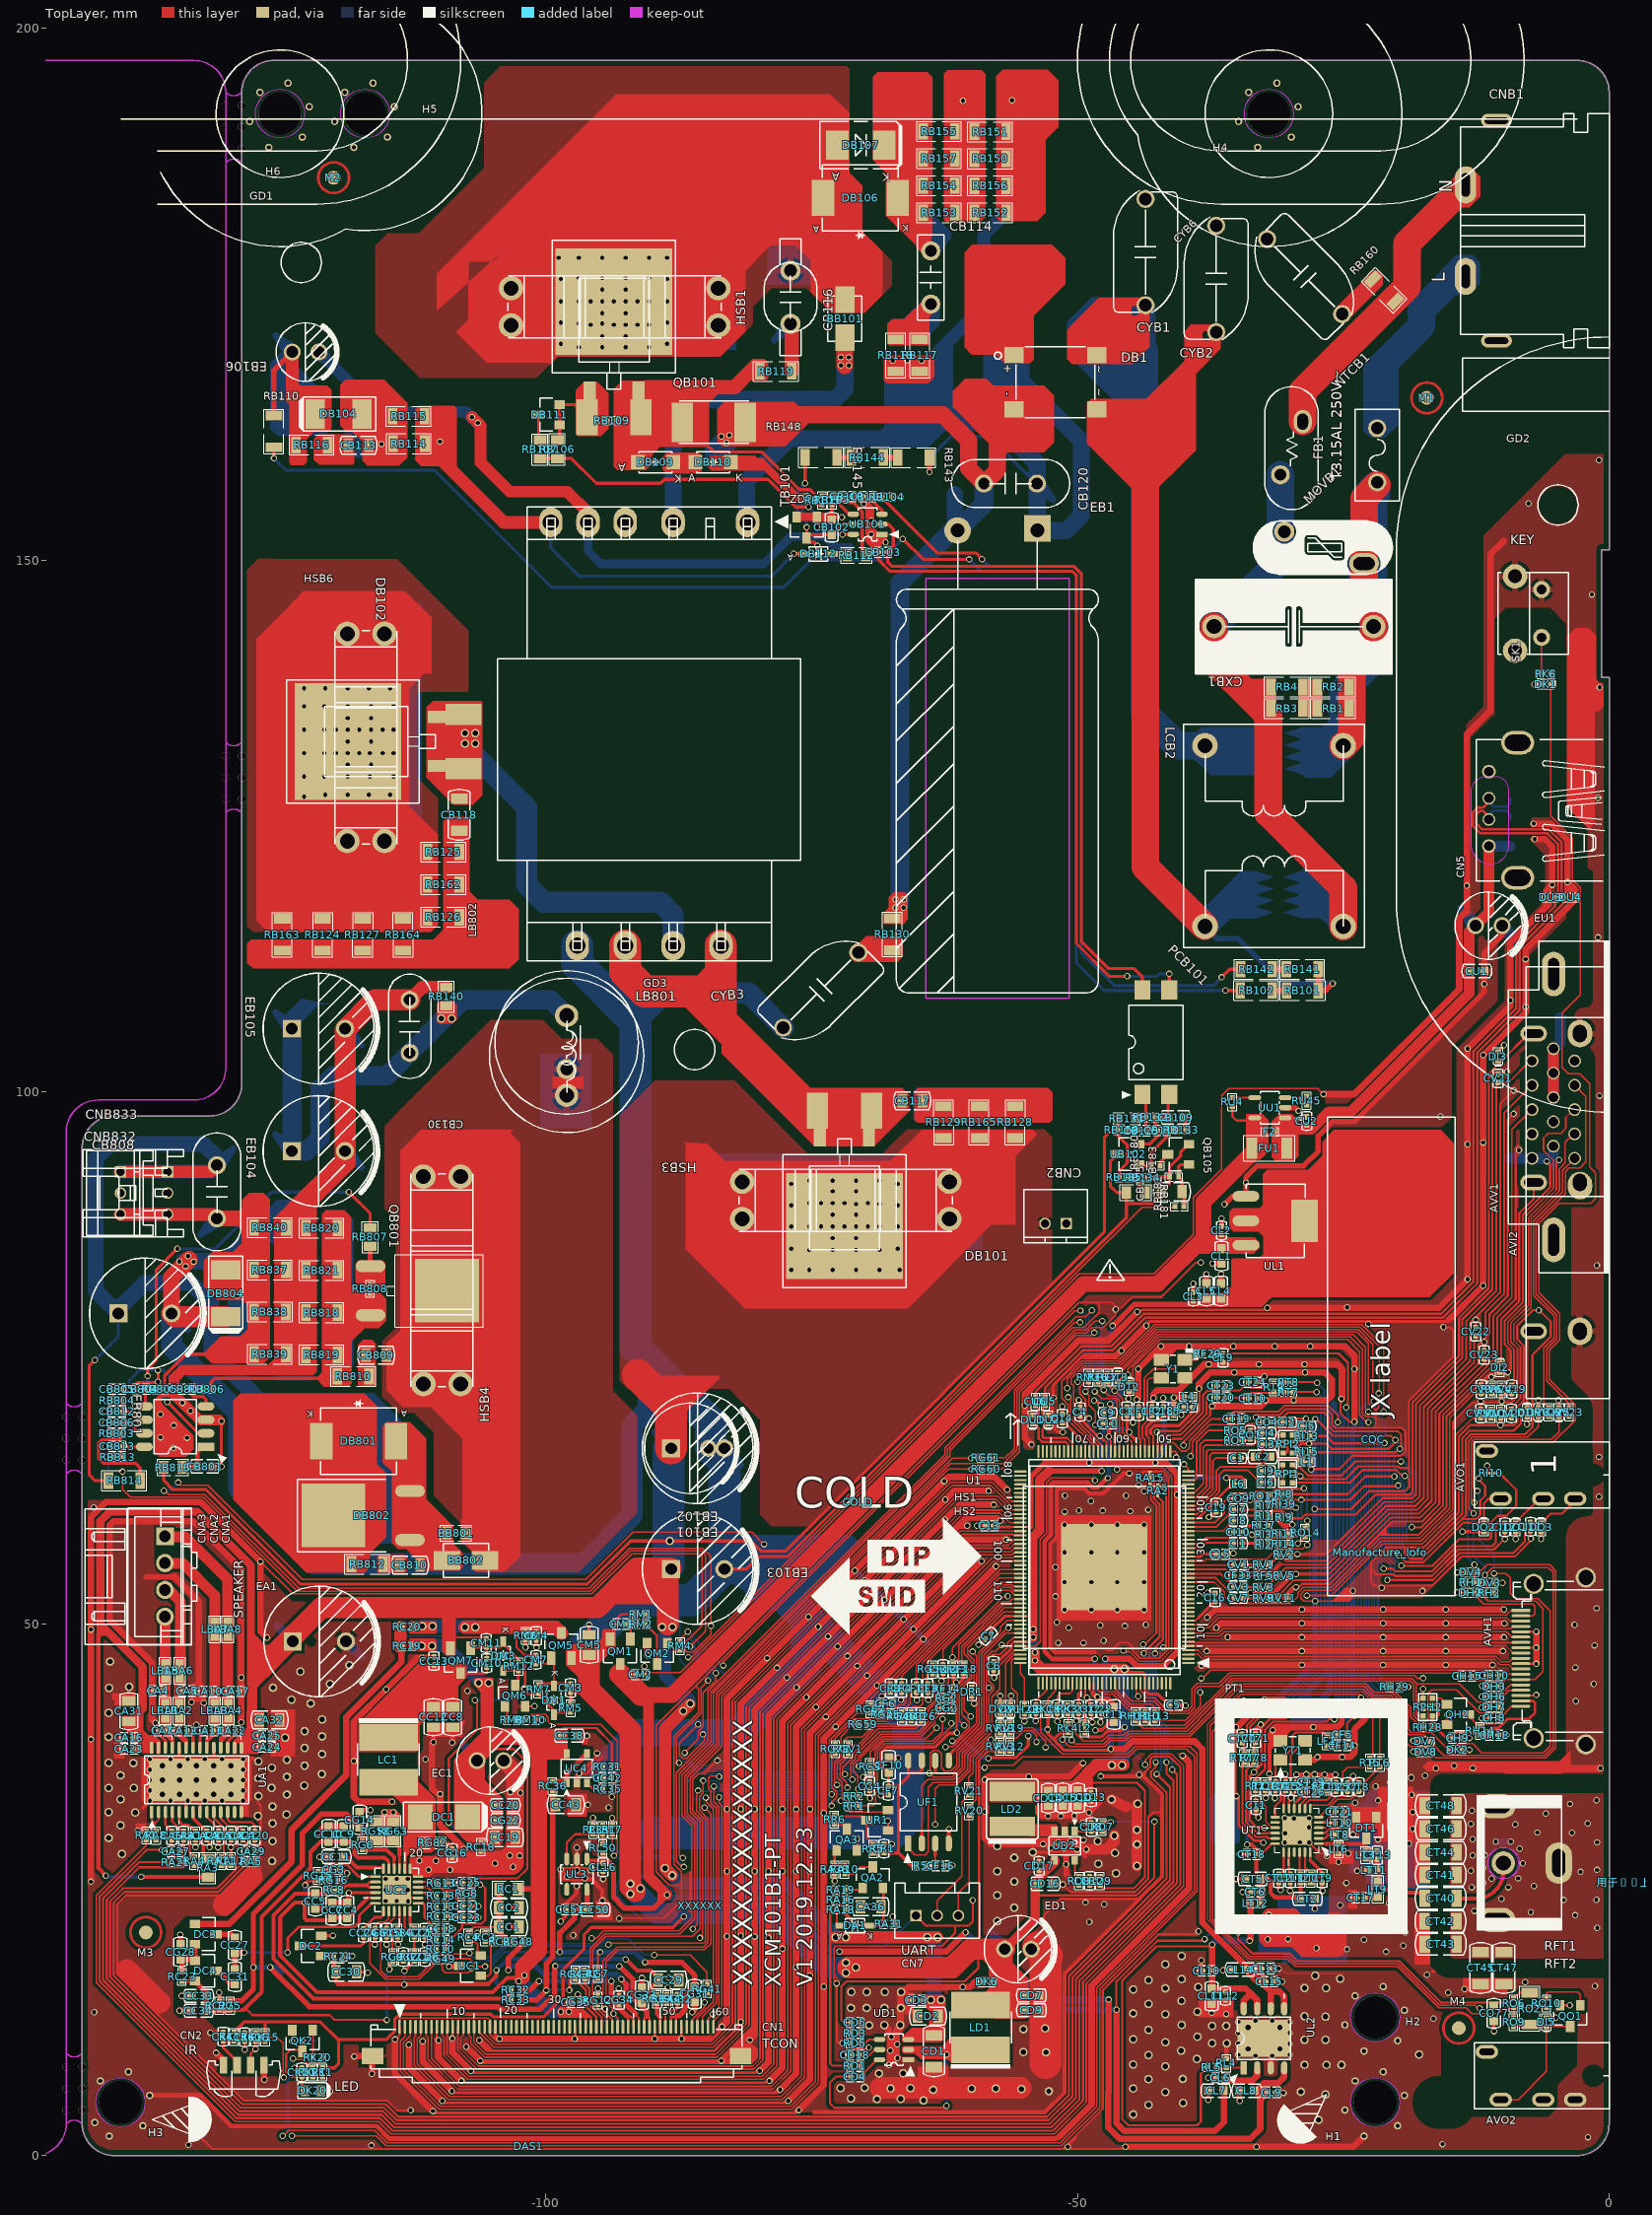
[diagram p0: TopLayer view]
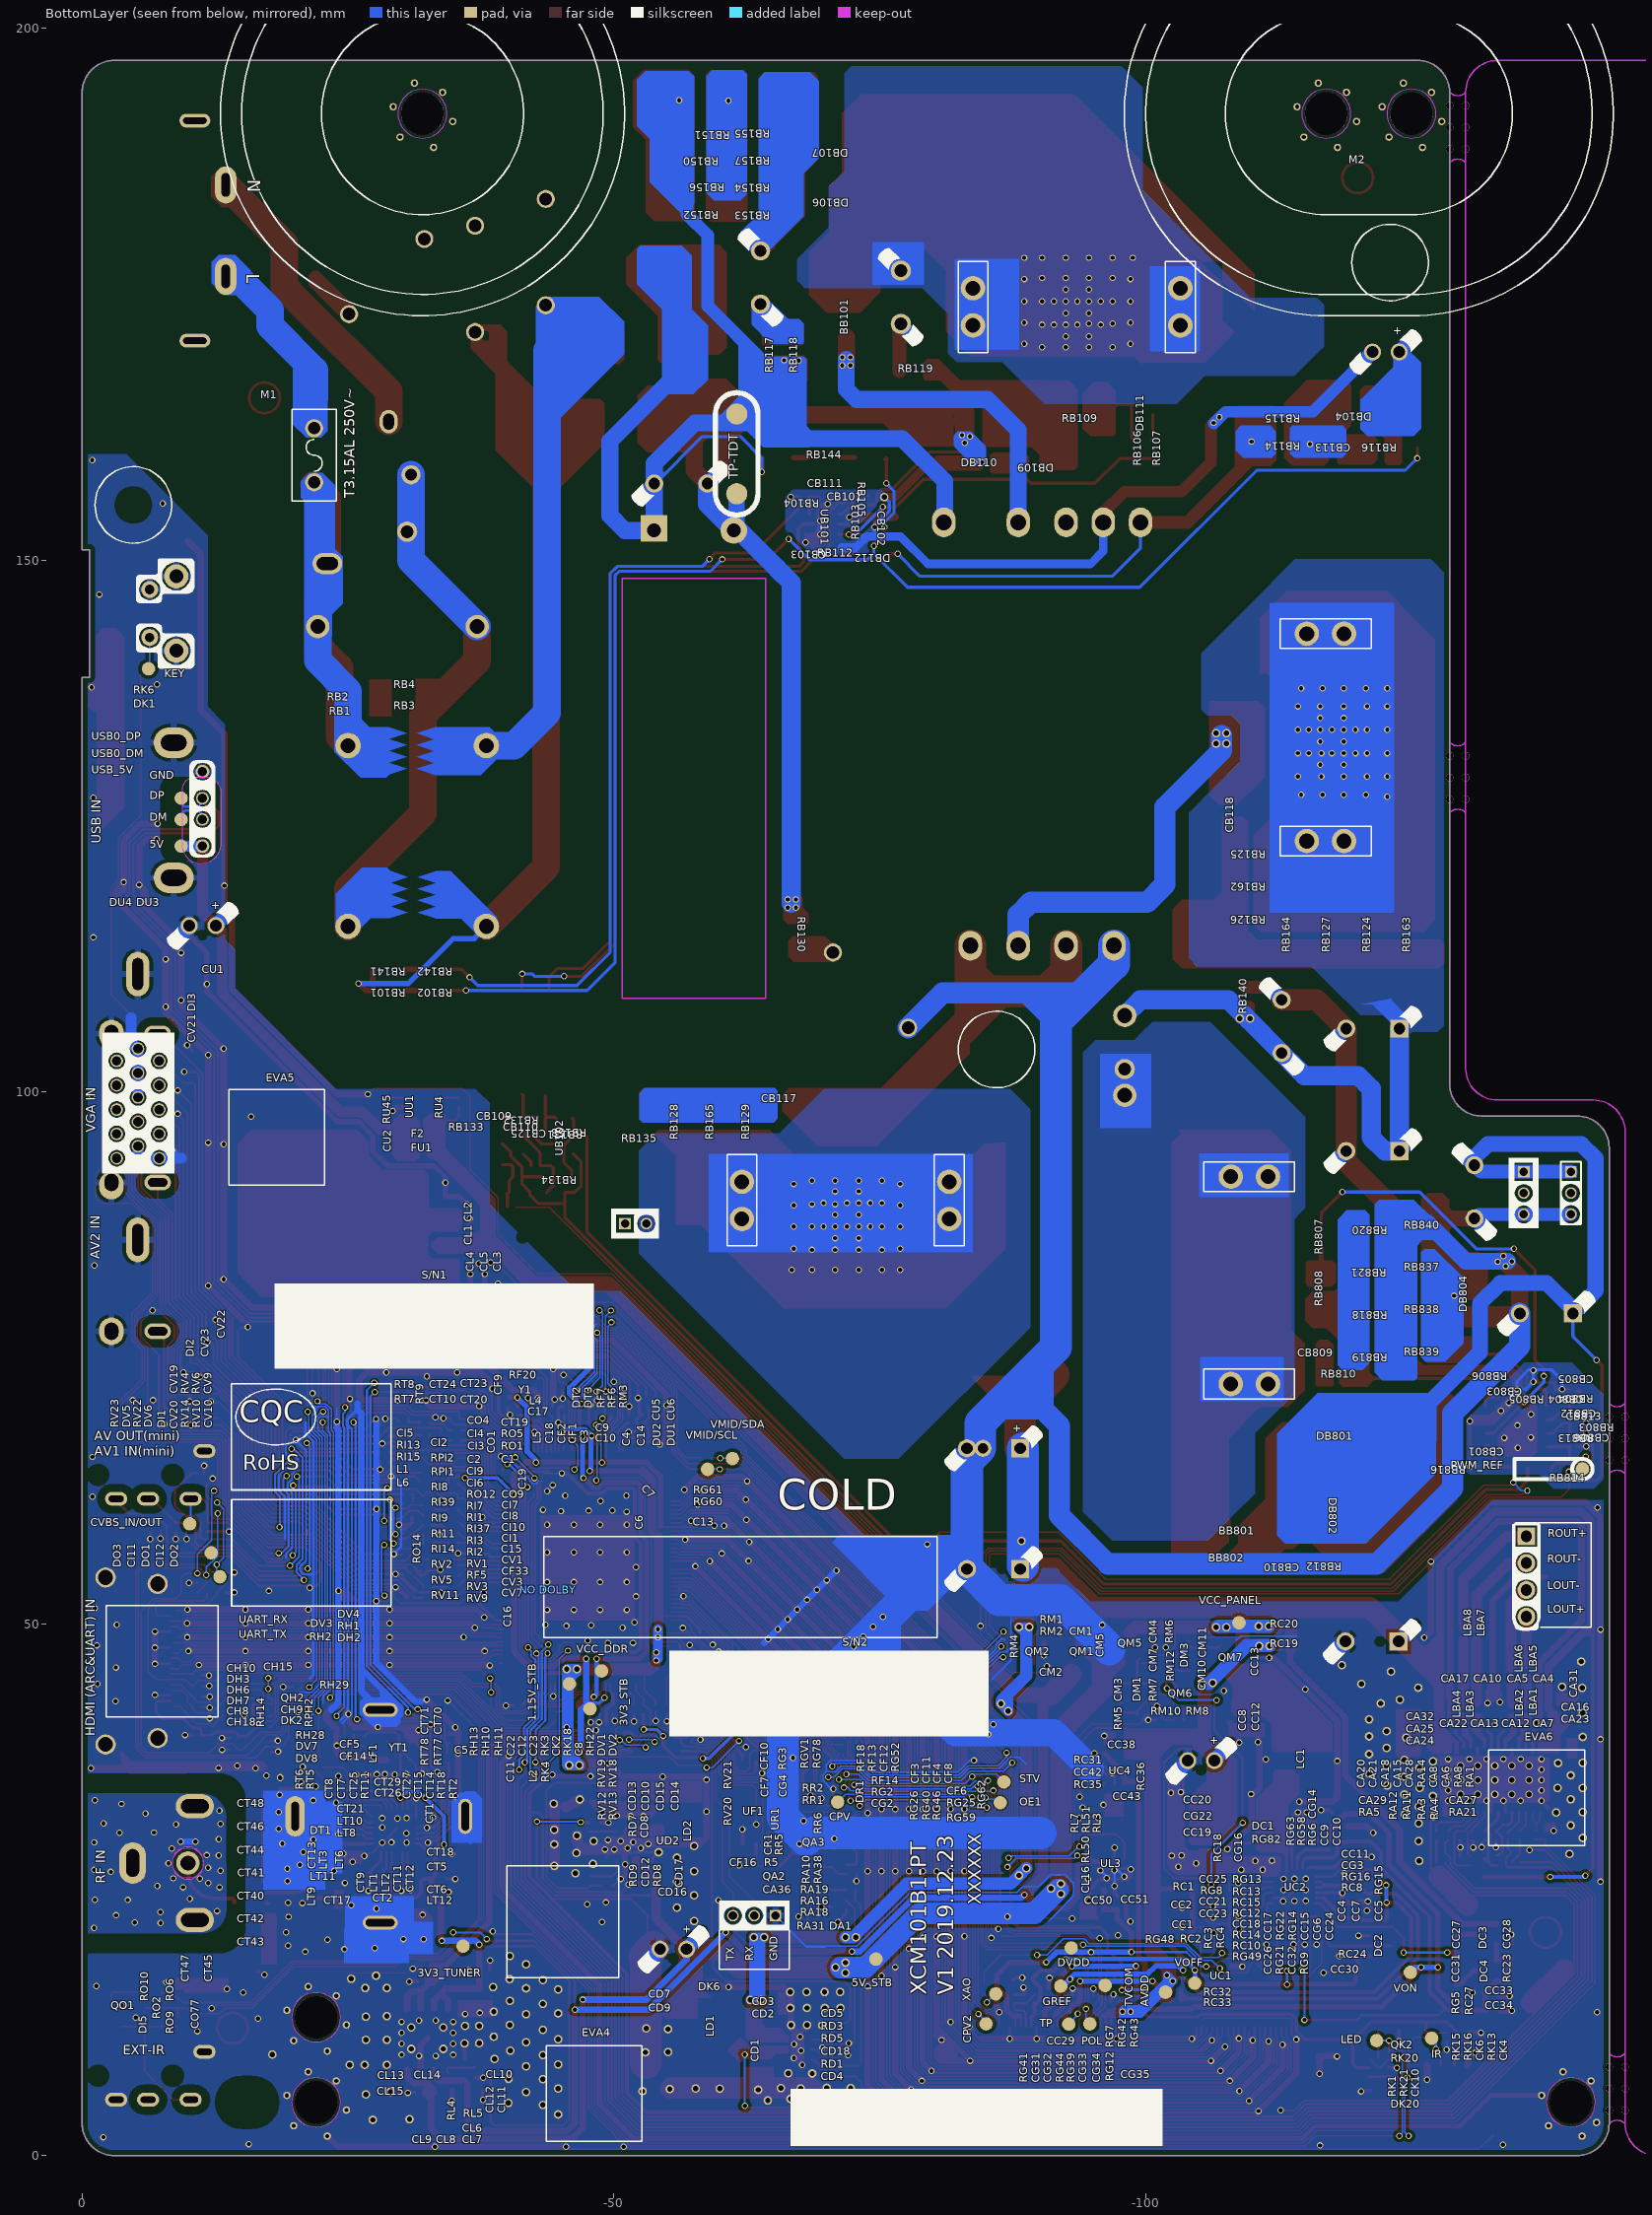
[diagram p1: BottomLayer view, seen from below]
# Altium PCB MISC86383-9.PcbDoc (part 1 of 18)
Units mm, origin at the board's own origin, x right, y up, seen from the top; angles counter-clockwise.
Board outline 143.6 x 197 mm, 2 copper layers (TopLayer, BottomLayer), stack 1.571 mm thick; 743 components, 401 nets, 2996 pads, 1077 vias.
Unrouted connection lines stored in the file: 4.

## Layer stack, top to bottom
TopSolder: solder mask 0.0102, Solder Resist, Dk 3.5
TopLayer: signal copper 0.0356
Dielectric1: core 1.5, FR-4, Dk 4.8
BottomLayer: signal copper 0.0356
BottomSolder: solder mask 0.0102, Solder Resist, Dk 3.5

## Board outline
-140.6,0 cw(c-140.6,3) -143.6,3 -143.6,94.75 cw(c-140.6,94.75) -140.6,97.75 -131.6,97.75 ccw(c-131.6,100.75) -128.6,100.75 -128.6,194 cw(c-125.6,194) -125.6,197 -3,197 cw(c-3,194) 0,194 0,151 -0.7,151 -0.7,139 0,139 0,3 cw(c-3,3) -3,0

## Design rules (kind name [scope] priority, off if disabled: settings)
Clearance ■KEEPOUT_18mil [(IsTrack Or IsArc) And (AsMM(Width) < 1) And IsKeepOut vs Not IsPad] p1: gap=0.457
Clearance ■HOT_8mm [InNetClass('HOT') vs InNetClass('All Nets') And (Not InNetClass('HOT'))] p2: gap=8
Clearance ■DFM_NPTH_10mil [(IsPadHoleValid And (PadIsPlated=false) Or IsPad And ((AsMM(PadXSize_AllLayers) < 1) or (AsMM(PadYSize_AllLayers) < 1 )) And IsKeepout) OR HasFootprintPad('ASSE*','0') vs Not IsPad] p3: gap=0.254
Clearance ■DFM_20mil [(IsTrack or IsArc or IsPad) And IsKeepOut vs IsTrack or IsArc or InPoly] p4: gap=0.508
Clearance ■C_RJ45_2mm [InNetClass('RJ45') vs Not InNetClass('RJ45') AND InNet('*')] p5: gap=2
Clearance ■VIA2VIA_6.2mil [(IsVia OR InPadClass('VIA5')) And Not ((IsVia OR InPadClass('VIA5')) And (AsMM(HoleDiameter) = 0.1)) vs (IsVia OR InPadClass('VIA5')) And Not ((IsVia OR InPadClass('VIA5')) And (AsMM(HoleDiameter) = 0.1))] p6: gap=0.157
Clearance ■V2V_BGA0p65_9p8mil [((IsVia OR InPadClass('VIA5')) And Not ((IsVia OR InPadClass('VIA5')) And (AsMM(HoleDiameter) = 0.1))) And (WithInRoom('BGA0p65-1') OR WithInRoom('BGA0p65-2')) vs ((IsVia OR InPadClass('VIA5')) And Not ((IsVia OR InPadClass('VIA5')) And (AsMM(HoleDiameter) = 0.1))) And (WithInRoom('BGA0p65-1') OR WithInRoom('BGA0p65-2'))] p7: gap=0.249
Clearance ■VIA2VIA_10.2mil [((IsVia OR InPadClass('VIA5')) And Not ((IsVia OR InPadClass('VIA5')) And (AsMM(HoleDiameter) = 0.1))) And Not (WithInRoom('BGA0p65-1') OR WithInRoom('BGA0p65-2')) vs ((IsVia OR InPadClass('VIA5')) And Not ((IsVia OR InPadClass('VIA5')) And (AsMM(HoleDiameter) = 0.1))) And Not (WithInRoom('BGA0p65-1') OR WithInRoom('BGA0p65-2'))] p8: gap=0.259
Clearance 0.3mm [(InNet('VGH') or InNet('*VGHM*')) and Not IsPad vs Not InPoly] p9: gap=0.3
Clearance ■PWR_A12_8mil [((InNetClass('PWR_A12_8mil') or InNet('*12V*') or InNet('*24V*') or InNet('AVDD') or InNet('*PVCC*') or InNet('*19V*') or InNet('*AMP*POWER*') or InNet('*AMP*VCC*') or InNet('*LNB*')) And Not InNetClass('A12_8mil_EXC')or InNet('VDD1')or InNet('VDD2')or InNet('CLK6')or InNet('CLK5')or InNet('CLK4')or InNet('CLK3')or InNet('CLK2')or InNet('CLK1')or InNet('DRVN')or InNet('DRVP')) and Not IsPad vs Not InPoly] p10: gap=0.203
Clearance ■PS_L2All_3.2mm [InNet('L-1') vs InNet('*')] p11: gap=3.2
Clearance ■PS_L2LN_1.5mm [InNet('L') Or InNet('L-2') Or InNet('L-3') Or InNet('L-4') Or InNet('L-5') Or InNet('L-6') vs InNet('L-N') And Not(InNet('L') Or InNet('L-2') Or InNet('L-3') Or InNet('L-4') Or InNet('L-5') Or InNet('L-6'))] p12: gap=1.5
Clearance ■PS_N2LN_1.5mm [InNet('N') OR InNet('N-1') OR InNet('N-2') OR InNet('N-3') OR InNet('N-4') OR InNet('N-5') OR InNet('N-6') vs InNet('L-N') And Not (InNet('N') OR InNet('N-1') OR InNet('N-2') OR InNet('N-3') OR InNet('N-4') OR InNet('N-5') OR InNet('N-6'))] p13: gap=1.5
Clearance ■PS_L2LN_3.1mm [InNet('L') Or InNet('L-2') Or InNet('L-3') Or InNet('L-4') Or InNet('L-5') Or InNet('L-6') vs InNet('*') And Not (InNet('L-N') Or InNet('L') Or InNet('L-2') Or InNet('L-3') Or InNet('L-4') Or InNet('L-5') Or InNet('L-6') Or OnLayer('KeepOutLayer'))] p14: gap=3.1
Clearance ■PS_N2LN_3.1mm [InNet('N') OR InNet('N-1') OR InNet('N-2') OR InNet('N-3') OR InNet('N-4') OR InNet('N-5') OR InNet('N-6') vs InNet('*') And Not (InNet('L-N') Or InNet('N') OR InNet('N-1') OR InNet('N-2') OR InNet('N-3') OR InNet('N-4') OR InNet('N-5') OR InNet('N-6') Or OnLayer('KeepOutLayer'))] p15: gap=3.1
Clearance 2.1mm [InNet('VBRIDGE')  Or InNet('D_QB101') vs InNet('*')And Not InNet('VBRIDGE')  And Not InNet('D_QB101')] p16: gap=2.1
Clearance 0.5mm [InNet('VBL')  Or InNet('LED+') Or InNet('D_QB801') vs InNet('*')And Not InNet('VBL')  And Not InNet('LED+')And Not InNet('D_QB801')] p17: gap=0.5
Clearance ■SIP2GND_8mil [HasFootprint('SIP*') vs InPoly] p18: gap=0.203
Clearance ■C_BGA_0P65 [HasFootprint('BGA*0.65*') vs InPoly] p19: gap=0.127
Clearance ■C_BGA_0P8 [HasFootprint('BGA*0.8*') vs InPoly] p20: gap=0.14
Clearance ■Poly_4mil [InPolygonClass('Poly_4mil') vs Not InPoly] p21: gap=0.102
Clearance ■Poly_5mil [InPolygonClass('Poly_5mil') vs Not InPoly] p22: gap=0.127
Clearance ■Poly_6.2mil [InPolygonClass('Poly_6.2mil') vs Not InPoly] p23: gap=0.157
Clearance Poly_7mil [InPolygonClass('Poly_7mil') vs Not InPoly] p24: gap=0.178
Clearance ■Poly_8mil [InPolygonClass('Poly_8mil') vs Not InPoly] p25: gap=0.203
Clearance ■C_RFGND_1.8mm [InNet('RFGND') vs Not (InNet('RF*IN*') OR((IsTrack Or IsArc) And (AsMils(Width) < 6) And IsKeepOut) OR InNet('NetCT28*'))] p26: gap=1.8
Clearance ■ESD_10mil [HasFootprint('*IEC*') Or HasFootprint('*-F1*') Or HasFootprint('ANT-RF*')] p27: gap=0.254
Clearance ■ESD_20mil [HasFootprint('*SHIELD*')] p28: gap=0.508
Clearance ■GND_12mil [InNet('GND') vs InPoly] p29: gap=0.305
Clearance ■ESD_30mil [(HasFootprint('SCART*') OR HasFootprint('AV*') OR HasFootprint('DB15*') OR HasFootprint('PHONE*')) vs OnBottomLayer] p30: gap=0.762
Clearance ■ESD_NT_30mil [HasFootprint('SCART*') Or HasFootprint('PHONE-HD-12') Or HasFootprint('PHONE-HD-17') Or HasFootprint('PHONE-HD-10') Or HasFootprint('PHONE-HD-26') vs InNet('GND') And OnTopLayer] p31: gap=0.762
Clearance ■DFM_TH_5mil [HasFootprint('GND') or HasFootprint('TP*') or HasFootprint('MARK*') or HasFootprint('SPARK_GAP') or HasFootprint('USB-HD-3-2') or HasFootprint('PHONE-HS-20') and Not IsRegion vs OnBottomlayer And IsPad OR IsPadHoleValid] p32: gap=0.127
Clearance ■DFM_HS60_5mil [InPadClass('HS60') vs InPadClass('HS60') OR IsPadHoleValid and not InPadClass('VIA5')] p33: gap=0.127
Clearance ■DFM_BCR_4mm [IsPadHoleValid vs IsBoardCutoutRegion] p34: gap=4
Clearance ■DFM_TH_4mm [OnBottomlayer And IsSMTPin vs IsPadHoleValid and not InPadClass('VIA5')] p35: gap=4
Clearance ■DFM_HS60_4mm [InPadClass('HS60') vs IsPad and OnBottomlayer] p36: gap=4
Clearance ■V2P_BGA0p65_4p7mil [HasFootprint('BGA*') and IsPad And (WithInRoom('BGA0p65-1') OR WithInRoom('BGA0p65-2')) vs (IsVia OR InPadClass('VIA5')) And Not (IsVia And (AsMM(HoleDiameter) = 0.1))] p37: gap=0.119
Clearance ■VIA2PAD_BGA_5mil [(HasFootprint('BGA*') and IsPad) And Not (WithInRoom('BGA0p65-1') OR WithInRoom('BGA0p65-2')) vs (IsVia OR InPadClass('VIA5')) And Not (IsVia And (AsMM(HoleDiameter) = 0.1))] p38: gap=0.127
Clearance ■VIA2PAD_6mil [(IsVia OR InPadClass('VIA5')) And Not ((IsVia OR InPadClass('VIA5')) And (AsMM(HoleDiameter) = 0.1)) vs IsPad And Not HasFootprintPad('*','EPAD') and Not HasFootprintPad('*','257') and Not HasFootprintPad('TP','*') and Not HasFootprintPad('GND','JP*') and Not HasFootprintPad('LQFP216/0.4-2','217') and Not HasFootprintPad('QFP16*','17') and Not HasFootprintPad('QFN16*','17') and Not HasFootprintPad('QFN20*','21') and Not HasFootprintPad('QFN24*','25') and Not HasFootprintPad( 'QFN24*','29') and Not HasFootprintPad('QFN28*','29') and Not HasFootprintPad('QFN32*','33') and Not HasFootprintPad('QFN36*','37') and Not HasFootprintPad('QFN36*','0') and Not HasFootprintPad('QFN32*','0') and Not HasFootprintPad('QFN40*','41') and Not HasFootprintPad('QFN48*','49') and Not HasFootprintPad('LQFP48/0.5-2','49') and Not HasFootprintPad('*SSOP32*','33') and Not HasFootprintPad('SOP8*','9') and Not HasFootprintPad('WSON8/1.27*','9') and Not HasFootprintPad('DFN10/0.5-1*','11') and Not HasFootprintPad('SON16/0.4','9') and Not HasFootprintPad('MSOP10/0.5-1','11') and Not HasFootprintPad('QFN56/0.5','57') and Not HasFootprintPad('LGA31/0.5','3*') and Not InPadClass('VIA_HS60') and Not HasFootprintPad('TSSOP16/0.65-3','17') and Not HasFootprintPad('QFP128/0.5-2','129') and Not HasFootprintPad('QFP128/0.4-5','129') and Not HasFootprintPad('PQFP48*','49') and Not HasFootprintPad('QFP156/0.4-1','157') and Not HasFootprintPad('D2PAK3-TO-252','2') and Not HasFootprintPad('D2PAK3','2') and Not HasFootprintPad('TO-252-GDS','D')  and Not HasFootprintPad('TO-252','2')  and Not HasFootprintPad('QFP156/0.4-2','157')] p39: gap=0.152
Clearance ■PAD2VIA5_6mil [(IsPad And Not (WithInRoom('BGA0p65-1') OR WithInRoom('BGA0p65-2'))) And ((AsMM(PadXSize_AllLayers) < 2.5) or ((AsMM(PadYSize_AllLayers) < 2.5))) And Not InPadclass('HS60') vs InPadClass('VIA5')] p40: gap=0.152
Clearance "■12mil for Polygon" [InPoly] p41: gap=0.305
Clearance 8mil [All] p42 off: gap=0.203
Clearance 7mil [All] p43 off: gap=0.178
Clearance 6.2mil [All] p44 off: gap=0.157
Clearance 6mil [All] p45 off: gap=0.152
Clearance 5.8mil [All] p46 off: gap=0.147
Clearance 5mil [Not ((IsTrack Or IsArc) And (Layer = 'KeepOutLayer')) vs Not (IsPad or ((IsTrack Or IsArc) And (Layer = 'KeepOutLayer')))] p47: gap=0.127
Clearance 4.5mil [Not ((IsTrack Or IsArc) And (Layer = 'KeepOutLayer')) vs Not (IsPad or ((IsTrack Or IsArc) And (Layer = 'KeepOutLayer')))] p48 off: gap=0.114
Clearance "4mil for Minimum" [Not ((IsTrack Or IsArc) And (Layer = 'KeepOutLayer')) vs Not (IsPad or ((IsTrack Or IsArc) And (Layer = 'KeepOutLayer')))] p49 off: gap=0.102
ComponentClearance ■DFMC_1mm [Not (InComponentClass('Co-Layout') Or HasFootprint('GND')) And (HasFootprint('T/E*') Or HasFootprint('T/PQ*') Or HasFootprint('USB*') Or HasFootprint('HDMI*') Or HasFootprint('USB*') Or HasFootprint('DC-*') Or HasFootprint('AV*') Or HasFootprint('ANT*') Or HasFootprint('PHONE*') Or HasFootprint('CICARD*') Or HasFootprint('CARD*') Or HasFootprint('DVI*') Or HasFootprint('DB*') Or HasFootprint('DP*') Or HasFootprint('DISPLAYPORT*') Or HasFootprint('OPTICAL*') Or HasFootprint('SCART*') Or HasFootprint('RJ45*') Or HasFootprint('USB*') Or HasFootprint('T-*') Or HasFootprint('T/*') Or HasFootprint('200-*') Or HasFootprint('ZhiJia*') Or HasFootprint('Dianpian*') Or HasFootprint('TanPian*') Or HasFootprint('P(*')) vs Not (InComponentClass('Co-Layout') Or HasFootprint('GND'))] p1 off: gap=1 collisioncheckmode=3 verticalgap=1 showdistances=FALSE
ComponentClearance ■DFMC_0.5mm [Not (InComponentClass('Co-Layout') Or HasFootprint('SO-23') Or HasFootprint('DIODE-s0402') Or HasFootprint('GND')) And (HasFootprint('M-*') Or HasFootprint('BGA*') Or HasFootprint('QFP*') Or HasFootprint('QFN*') Or HasFootprint('*DFN*') Or HasFootprint('*SOP*') Or HasFootprint('LGA*') Or HasFootprint('SOIC*') Or HasFootprint('EC*') Or HasFootprint('AC-*') Or HasFootprint('DIODE*') Or HasFootprint('XTAL*') Or HasFootprint('SO-*') Or HasFootprint('L/LC*') Or HasFootprint('L(*') Or HasFootprint('WIFI*') Or HasFootprint('SATA*') Or HasFootprint('POGO*') Or HasFootprint('SOT-223') Or HasFootprint('TO-252') Or HasFootprint('TO-263') Or HasFootprint('KEY*') Or HasFootprint('SW*') Or HasFootprint('DIP*') Or HasFootprint('SIP*') Or HasFootprint('DIP*') Or HasFootprint('CON*') Or HasFootprint('FFC*') Or HasFootprint('FPC*') Or HasFootprint('GDT*') Or HasFootprint('R2512*') Or HasFootprint('R2725*') Or HasFootprint('L2012*') Or HasFootprint('L2520*')) vs Not (InComponentClass('Co-Layout') Or HasFootprint('SO-23') Or HasFootprint('DIODE-s0402') Or HasFootprint('GND'))] p2 off: gap=0.5 collisioncheckmode=3 verticalgap=0.5 showdistances=FALSE
ComponentClearance ■DFMC_0.4mm [Not (InComponentClass('Co-Layout') Or HasFootprint('GND')) And (HasFootprint('C0201*') Or HasFootprint('C0402*') Or HasFootprint('C0603*') Or HasFootprint('C0805*') Or HasFootprint('C1206*') Or HasFootprint('C1210*') Or HasFootprint('R0201*') Or HasFootprint('R0402*') Or HasFootprint('R0603*') Or HasFootprint('R0805*') Or HasFootprint('R*0402*') Or HasFootprint('L0201*') Or HasFootprint('L0402*') Or HasFootprint('L0603*') Or HasFootprint('L0805*') Or HasFootprint('L1206*') Or HasFootprint('DIODE-s0402')) vs Not (InComponentClass('Co-Layout') Or HasFootprint('GND')) And (HasFootprint('C0201*') Or HasFootprint('C0402*') Or HasFootprint('C0603*') Or HasFootprint('C0805*') Or HasFootprint('C1206*') Or HasFootprint('C1210*') Or HasFootprint('R0201*') Or HasFootprint('R0402*') Or HasFootprint('R0603*') Or HasFootprint('R0805*') Or HasFootprint('R*0402*') Or HasFootprint('L0201*') Or HasFootprint('L0402*') Or HasFootprint('L0603*') Or HasFootprint('L0805*') Or HasFootprint('L1206*') Or HasFootprint('DIODE-s0402'))] p3 off: gap=0.4 collisioncheckmode=3 verticalgap=0.4 showdistances=FALSE
ComponentClearance ■DFMC_0.36mm [Not (InComponentClass('Co-Layout') Or HasFootprint('GND')) And HasFootprint('R1206*') vs Not (InComponentClass('Co-Layout') Or HasFootprint('GND')) And HasFootprint('R1206*')] p4 off: gap=0.36 collisioncheckmode=3 verticalgap=0.36 showdistances=FALSE
ComponentClearance ■DFMC_0.25mm [Not (InComponentClass('Co-Layout') Or HasFootprint('GND')) vs Not (InComponentClass('Co-Layout') Or HasFootprint('GND'))] p5 off: gap=0.25 collisioncheckmode=3 verticalgap=0.25 showdistances=FALSE
DiffPairsRouting ■DiffPair_USB_DiffPairsRouting [InDifferentialPairClass('USB')] p1: maxlimit=0.127 minlimit=0.102 mostfreqgap=0.127 toplayer_minwidth=0.381 toplayer_maxwidth=0.381 toplayer_prefwidth=0.381 bottomlayer_minwidth=0.381 bottomlayer_maxwidth=0.381 bottomlayer_prefwidth=0.381 maxuncoupledlength=5.08
DiffPairsRouting ■DiffPair_LVDS_DiffPairsRouting [InDifferentialPairClass('LVDS')] p2: maxlimit=0.127 minlimit=0.102 mostfreqgap=0.127 toplayer_minwidth=0.381 toplayer_maxwidth=0.381 toplayer_prefwidth=0.381 bottomlayer_minwidth=0.381 bottomlayer_maxwidth=0.381 bottomlayer_prefwidth=0.381 maxuncoupledlength=12.7
DiffPairsRouting ■DiffPair_HDMI_DiffPairsRouting [InDifferentialPairClass('HDMI')] p3: maxlimit=0.127 minlimit=0.102 mostfreqgap=0.127 toplayer_minwidth=0.381 toplayer_maxwidth=0.381 toplayer_prefwidth=0.381 bottomlayer_minwidth=0.381 bottomlayer_maxwidth=0.381 bottomlayer_prefwidth=0.381 maxuncoupledlength=5.08
DiffPairsRouting [All] p4: maxlimit=0.254 minlimit=0.254 mostfreqgap=0.254 toplayer_minwidth=0.381 toplayer_maxwidth=0.381 toplayer_prefwidth=0.381 bottomlayer_minwidth=0.381 bottomlayer_maxwidth=0.381 bottomlayer_prefwidth=0.381 maxuncoupledlength=12.7
FabricationTestPointUsage TestPointUsage [All] p1: valid=0 allowmultiple=FALSE
FabricationTestpoint Testpoint [All] p1: side=3 testpointundercomponent=TRUE minsize=1.016 maxsize=2.54 preferedsize=1.524 minholesize=0.508 maxholesize=1.016 preferedholesize=0.813 testpointgrid=0.025 allowsidetop=TRUE allowsidebottom=TRUE usegrid=TRUE gridtolerance=0
HoleSize HoleSize_VIA [ISVIA] p1 off: absolutevalues=TRUE maxlimit=0.6 minlimit=0.2 maxpercent=80.000 minpercent=20.000
HoleToHoleClearance Hole2Hole [All] p1 off: gap=0.457 allowstackedmicrovias=FALSE
MatchedLengths DiffPair_USB_MatchedLengths [InDifferentialPairClass('USB')] p1: tolerance=2.54 checknetsindiffpair=TRUE checkdiffpairvsdiffpair=TRUE checkothers=TRUE
MatchedLengths DiffPair_LVDS_MatchedLengths [InDifferentialPairClass('LVDS')] p2: tolerance=2.54 checknetsindiffpair=TRUE checkdiffpairvsdiffpair=TRUE checkothers=TRUE
MatchedLengths DiffPair_HDMI_MatchedLengths [InDifferentialPairClass('HDMI')] p3: tolerance=2.54 checknetsindiffpair=TRUE checkdiffpairvsdiffpair=TRUE checkothers=TRUE
MinimumAnnularRing [All] p1: minimumring=0.1
MinimumSolderMaskSliver ■MiniSolderMaskSliver [All] p1 off: minsoldermaskwidth=0.098
NetAntennae [Not (HasFootprint('ANT-7') or HasFootprint('ANT-BLUECORE'))] p1: netantennaetolerance=1.016
PermittedLayers [All] p1: toplayerpermitted=TRUE bottomlayerpermitted=TRUE
PlaneClearance ■Plane_ESD_30mil [(HasFootprint('SCART*') OR HasFootprint('AV*') OR HasFootprint('DB15*') OR HasFootprint('PHONE*'))] p1: clearance=0.762
PlaneClearance ■Plane_All_9mil [All] p2: clearance=0.229
PlaneConnect ■PlaneOverAll [IsVia or InPadClass('VIA5') Or HasFootprint('ASSE*') OR InPadclass('HS60')] p1: planeconnectstyle=Direct reliefexpansion=0.508 reliefentries=4 reliefconductorwidth=0.254 reliefairgap=0.254
PlaneConnect ■PlaneConnect [All] p2: planeconnectstyle=Relief reliefexpansion=0.305 reliefentries=4 reliefconductorwidth=0.762 reliefairgap=0.305
PolygonConnect ■PourOverAll [IsVia Or InPadclass('HS60') Or InPadClass('VIA5') Or HasFootprint('ASSE*') Or HasFootprint('DIODE-S0402') Or HasFootprint('RCL0524P') Or HasFootprint('SOT-89') OR HasFootprint('SOT-223') OR HasFootprint('TO-252') OR HasFootprint('TO-263') OR HasFootprint('DIODE') OR HasFootprint('SW-HS-2') OR HasFootprint('HDMI*') OR HasFootprint('SO-8B') OR HasFootprint('GND') OR HasFootprint('PHONE*') OR HasFootprint('DIP18/2.54-2') OR HasFootprint('DIP18/2.54-1') OR HasFootprint('UFL-R-SMT-1') OR HasFootprint('WIFI') OR HasFootprint('UM02BS') OR HasFootprint('*SCART*') OR HasFootprint('TSOT23-8/0.65') OR HasFootprint('*SOT-23-*') OR HasFootprint('SOP23-5-1') OR HasFootprint('SOP6/0.95') OR HasFootprint('M-WIFI-2-M603USA1') OR HasFootprint('M-MT7632U') OR HasFootprint('SOP8/1.27') OR HasFootprint('SOP8/1.27-3') OR HasFootprint('TSOT23-6') vs IsPolygon] p1: connectstyle=Direct reliefconductorwidth=0.254 reliefentries=4 polygonreliefangle="90 Angle" airgapwidth=0.254
PolygonConnect ■BGA_0P65 [HasFootprint('BGA*0.65*') vs IsPoly] p2: connectstyle=Relief reliefconductorwidth=0.203 reliefentries=4 polygonreliefangle="45 Angle" airgapwidth=0.254
PolygonConnect ■BGA_0P8 [HasFootprint('BGA*0.8*') vs IsPoly] p3: connectstyle=Relief reliefconductorwidth=0.229 reliefentries=4 polygonreliefangle="45 Angle" airgapwidth=0.254
PolygonConnect ■Polygon_RFGND [InNet('RFGND')] p4: connectstyle=Direct reliefconductorwidth=0.254 reliefentries=4 polygonreliefangle="90 Angle" airgapwidth=0.254
PolygonConnect ■ESD_SCART [HasFootprint('SCART*') vs IsPolygon And onBottomlayer] p5: connectstyle=Direct reliefconductorwidth=0.762 reliefentries=4 polygonreliefangle="90 Angle" airgapwidth=0.254
PolygonConnect ■C2Polygon_35mil [HasFootprint('EC*') vs IsPolygon] p6: connectstyle=Relief reliefconductorwidth=0.889 reliefentries=4 polygonreliefangle="90 Angle" airgapwidth=0.254
PolygonConnect ■C2Polygon_30mil [(HasFootprint('*0805*') OR HasFootprint('*1206*')) vs IsPolygon] p7: connectstyle=Relief reliefconductorwidth=0.762 reliefentries=4 polygonreliefangle="90 Angle" airgapwidth=0.254
PolygonConnect ■C2Polygon_25mil [HasFootprint('*0603*') Or IsThruPin vs IsPolygon] p8: connectstyle=Relief reliefconductorwidth=0.635 reliefentries=4 polygonreliefangle="90 Angle" airgapwidth=0.254
PolygonConnect ■C2Polygon_12mil [IsSMTPin vs IsPolygon] p9: connectstyle=Relief reliefconductorwidth=0.305 reliefentries=4 polygonreliefangle="90 Angle" airgapwidth=0.254
RoutingVias 0.6_0.4 [All] p1: holewidth=0.4 width=0.6 viastyle="Through Hole" minholewidth=0.4 minwidth=0.6 maxholewidth=0.4 maxwidth=0.6
RoutingVias 0.8_0.5 [All] p2 off: holewidth=0.5 width=0.8 viastyle="Through Hole" minholewidth=0.5 minwidth=0.8 maxholewidth=0.5 maxwidth=0.8
RoutingVias 0.5_0.3 [All] p3 off: holewidth=0.3 width=0.5 viastyle="Through Hole" minholewidth=0.3 minwidth=0.5 maxholewidth=0.3 maxwidth=0.5
RoutingVias 0.45_0.25 [All] p4 off: holewidth=0.25 width=0.45 viastyle="Through Hole" minholewidth=0.25 minwidth=0.45 maxholewidth=0.25 maxwidth=0.45
RoutingVias 0.4_0.2 [All] p5 off: holewidth=0.2 width=0.4 viastyle="Through Hole" minholewidth=0.2 minwidth=0.4 maxholewidth=0.2 maxwidth=0.4
RoutingVias 0.25_0.1 [All] p6 off: holewidth=0.1 width=0.25 viastyle="Through Hole" minholewidth=0.1 minwidth=0.25 maxholewidth=0.1 maxwidth=0.25
SMDNeckDown ■SMDNeckDown_Chip [HasFootprint('FFC*') or HasFootprint('QFP*') or HasFootprint('QFN*') or HasFootprint('HDMI*') or HasFootprint('BGA*')] p1: percent=100.000
SMDToCorner [All] p1 off: distance=40000
ShortCircuit ■ShortCircuit_JP [HasFootprintPad( 'GND','JP_1K') vs HasFootprintPad( 'GND','JP_2K')] p1: allowed=TRUE
ShortCircuit ■ShortCircuit_ViaOnEpad [HasFootprintPad( '*','EPAD') vs IsVia AND InNet('*')] p2: allowed=TRUE
ShortCircuit ■ShortCircuit_R0402 [HasFootprintPad('R0402SC','1') OR HasFootprintPad('R0402SC','2') vs HasFootprintPad('R0402SC','3')] p3: allowed=TRUE
ShortCircuit ■ShortCircuit_RP2_0402 [HasFootprintPad('RP2*0402-1SC','1') OR HasFootprintPad('RP2*0402-1SC','2') vs HasFootprintPad('RP2*0402-1SC','5')] p4: allowed=TRUE
ShortCircuit ■ShortCircuit_RP2-0402 [HasFootprintPad('RP2*0402-1SC','3') OR HasFootprintPad('RP2*0402-1SC','4') vs HasFootprintPad('RP2*0402-1SC','6')] p5: allowed=TRUE
ShortCircuit ■ShortCircuit_LC4_SC1 [HasFootprintPad('L/LC4/0.85*0.65SC','1') OR HasFootprintPad('L/LC4/0.85*0.65SC','2') vs HasFootprintPad('L/LC4/0.85*0.65SC','5')] p6: allowed=TRUE
ShortCircuit ■ShortCircuit_LC4-SC1 [HasFootprintPad('L/LC4/0.85*0.65SC','3') OR HasFootprintPad('L/LC4/0.85*0.65SC','4') vs HasFootprintPad('L/LC4/0.85*0.65SC','5')] p7: allowed=TRUE
ShortCircuit ■ShortCircuit_R0603 [HasFootprintPad('R0603SC','1') OR HasFootprintPad('R0603SC','2') vs HasFootprintPad('R0603SC','3')] p8: allowed=TRUE
ShortCircuit ■ShortCircuit_R0805 [HasFootprintPad('R0805SC','1') OR HasFootprintPad('R0805SC','2') vs HasFootprintPad('R0805SC','3')] p9: allowed=TRUE
ShortCircuit ■ShortCircuit_L0805 [HasFootprintPad('L0805SC','1') OR HasFootprintPad('L0805SC','2') vs HasFootprintPad('L0805SC','3')] p10: allowed=TRUE
ShortCircuit ■ShortCircuit_R1206 [HasFootprintPad('R1206SC','1') OR HasFootprintPad('R1206SC','2') vs HasFootprintPad('R1206SC','3')] p11: allowed=TRUE
ShortCircuit ■ShortCircuit [InNet('*')] p12: allowed=FALSE
SilkToSilkClearance ■Silk2Silk [All] p1: silktosilkclearance=0.127
SilkToSolderMaskClearance ■SilkOverPads [IsText] p1: minsilkscreentomaskgap=0.003 clearancetoexposedcopper=TRUE
SolderMaskExpansion ■SolderMask_VIA [IsVia] p1: expansion=0.13
SolderMaskExpansion ■SolderMask_All [All] p2: expansion=0.051
UnRoutedNet ■UnRoutedNet [All] p1:
ViasUnderSMD [All] p1: allowed=FALSE
Width ■Width_2.5mm [InFromToClass('Width_2.5mm')] p1: maxlimit=2.5 minlimit=2.5 preferedwidth=2.5
Width ■Width_1.5mm [InFromToClass('Width_1.5mm')] p2: maxlimit=1.5 minlimit=1.5 preferedwidth=1.5
Width ■DiffPair_USB_Width [InDifferentialPairClass('USB')] p3: maxlimit=0.279 minlimit=0.102 preferedwidth=0.279
Width ■DiffPair_LVDS_Width [InDifferentialPairClass('LVDS')] p4: maxlimit=0.178 minlimit=0.102 preferedwidth=0.178
Width ■DiffPair_HDMI_Width [InDifferentialPairClass('HDMI')] p5: maxlimit=0.178 minlimit=0.102 preferedwidth=0.178
Width [All] p6: maxlimit=12.7 minlimit=0.076 preferedwidth=0.203
16 further rules are at their usual default settings.

## Classes and differential pairs
pad class VIA5: Free-VIA5
polygon class Poly_5mil: 5
component class PCB_info: AI_V COLD CQC DAS1 H1 H2 H3 H4 H5 H6 M3 M4 M5 M6 MAC Manufacture_Info QR1 QR2 S/N1 S/N2
component class SCH_info: HS1 HS2 "NO DOLBY" XCM101B1-PT XXXXXX XXXXXXXXXXXXXXX XXXX丝印待提供 用于U1上
component class TV#01_POWER: 1.15V_STB 3V3_STB 3V3_TUNER 5V_STB CA36 CD1 CD2 CD3 CD4 CD5 CD7 CD8 CD9 CD10 CD12 CD13 CD14 CD15 CD16 CD17 CD18 CG2 CG4 CL1 CL2 CL3 CL4 CL5 CL6 CL7 CL8 CL9 CL10 CL11 CL12 CL13 CL14 CL15 CM1 CM2 CM3 CM4 CM5 CM7 DA1 DK6 DM1 ED1 LD1 LD2 QA2 QA3 QM1 QM2 QM5 QM6 RA10 RA16 RA18 RA19 RA31 RA38 RD1 RD3 RD5 RD7 RD8 RD9 RG2 RG3 RL2 RL4 RL5 RM1 RM2 RM3 RM4 RM5 RM6 RM7 RM8 RM10 UD1 UD2 UL1 UL2 VCC_DDR VCC_PANEL
component class TV#02_TSU69ZBT: C1 C2 C3 C4 C5 C6 C7 C8 C9 C10 C11 C12 C13 C14 C15 C16 C17 C18 C19 C22 C23 CF1 CF2 CF3 CF4 CF5 CF6 CF7 CF8 CF9 CF10 CF11 CF12 CF14 CF16 CI7 CI10 CN7 CR1 DR1 DV1 DV2 DV5 DV6 DV7 DV8 L1 L2 L4 L5 L6 LF1 R5 RF6 RF7 RF13 RF14 RF18 RF20 RH22 RI7 RI8 RI10 RI11 RI37 RI39 RR1 RR2 RR5 RR6 RV12 RV13 RV18 RV19 RV20 RV21 U1 UART_RX UART_TX UF1 UR1 Y1
component class TV#03_INPUT: AVI2 AVO1 AVO2 AVV1 CF33 CI1 CI2 CI3 CI4 CI5 CI6 CI8 CI9 CI11 CI12 CN5 CO1 CO4 CO9 CO77 CU1 CU2 CU5 CU6 CV1 CV3 CV7 CV9 CV10 CV19 CV20 CV21 CV22 CV23 CVBS_IN/OUT DI1 DI2 DI3 DI5 DO1 DO2 DO3 DU1 DU2 DU3 DU4 DV3 DV4 EU1 F1 F2 FU1 QO1 RF5 RI1 RI2 RI3 RI9 RI13 RI14 RI15 RO1 RO2 RO5 RO6 RO9 RO10 RO12 RO14 RPI1 RPI2 RU4 RU45 RV1 RV2 RV3 RV4 RV5 RV6 RV9 RV10 RV11 RV14 RV22 RV23 USB0_DM USB0_DP USB_5V UU1
component class TV#04_HDMI(UART&CEC&ARC): AVH1 CH8 CH9 CH10 CH15 CH18 DH2 DH3 DH6 DH7 QH2 RH1 RH2 RH10 RH11 RH13 RH14 RH28 RH29 RPH2
component class TV#05_AMP: CA4 CA5 CA6 CA7 CA8 CA10 CA12 CA13 CA15 CA16 CA17 CA18 CA20 CA21 CA22 CA23 CA24 CA25 CA27 CA28 CA29 CA31 CA32 CNA1 CNA2 CNA3 EA1 LBA1 LBA2 LBA3 LBA4 LBA5 LBA6 LBA7 LBA8 RA1 RA2 RA3 RA4 RA5 RA8 RA11 RA12 RA14 RA15 RA21 UA1
component class TV#06_R842-V69T&MSD3553T&V56T: CT1 CT2 CT5 CT6 CT7 CT8 CT9 CT10 CT11 CT12 CT13 CT14 CT15 CT17 CT18 CT19 CT20 CT21 CT23 CT24 CT25 CT26 CT27 CT29 CT40 CT41 CT42 CT43 CT44 CT45 CT46 CT47 CT48 CT70 CT71 DT1 DT2 DT3 GDT1 GDT2 LT1 LT2 LT3 LT6 LT8 LT9 LT10 LT11 LT12 PT1 RFT1 RFT2 RT2 RT5 RT6 RT7 RT8 RT9 RT11 RT18 RT77 RT78 UT1 YT1
component class TV#07_KEY&IR&LED: CK2 CK4 CK6 CK10 CN2 DK1 DK2 DK20 IR KEY LED QK2 RK1 RK3 RK4 RK6 RK13 RK15 RK16 RK18 RK20 RK21 SK1